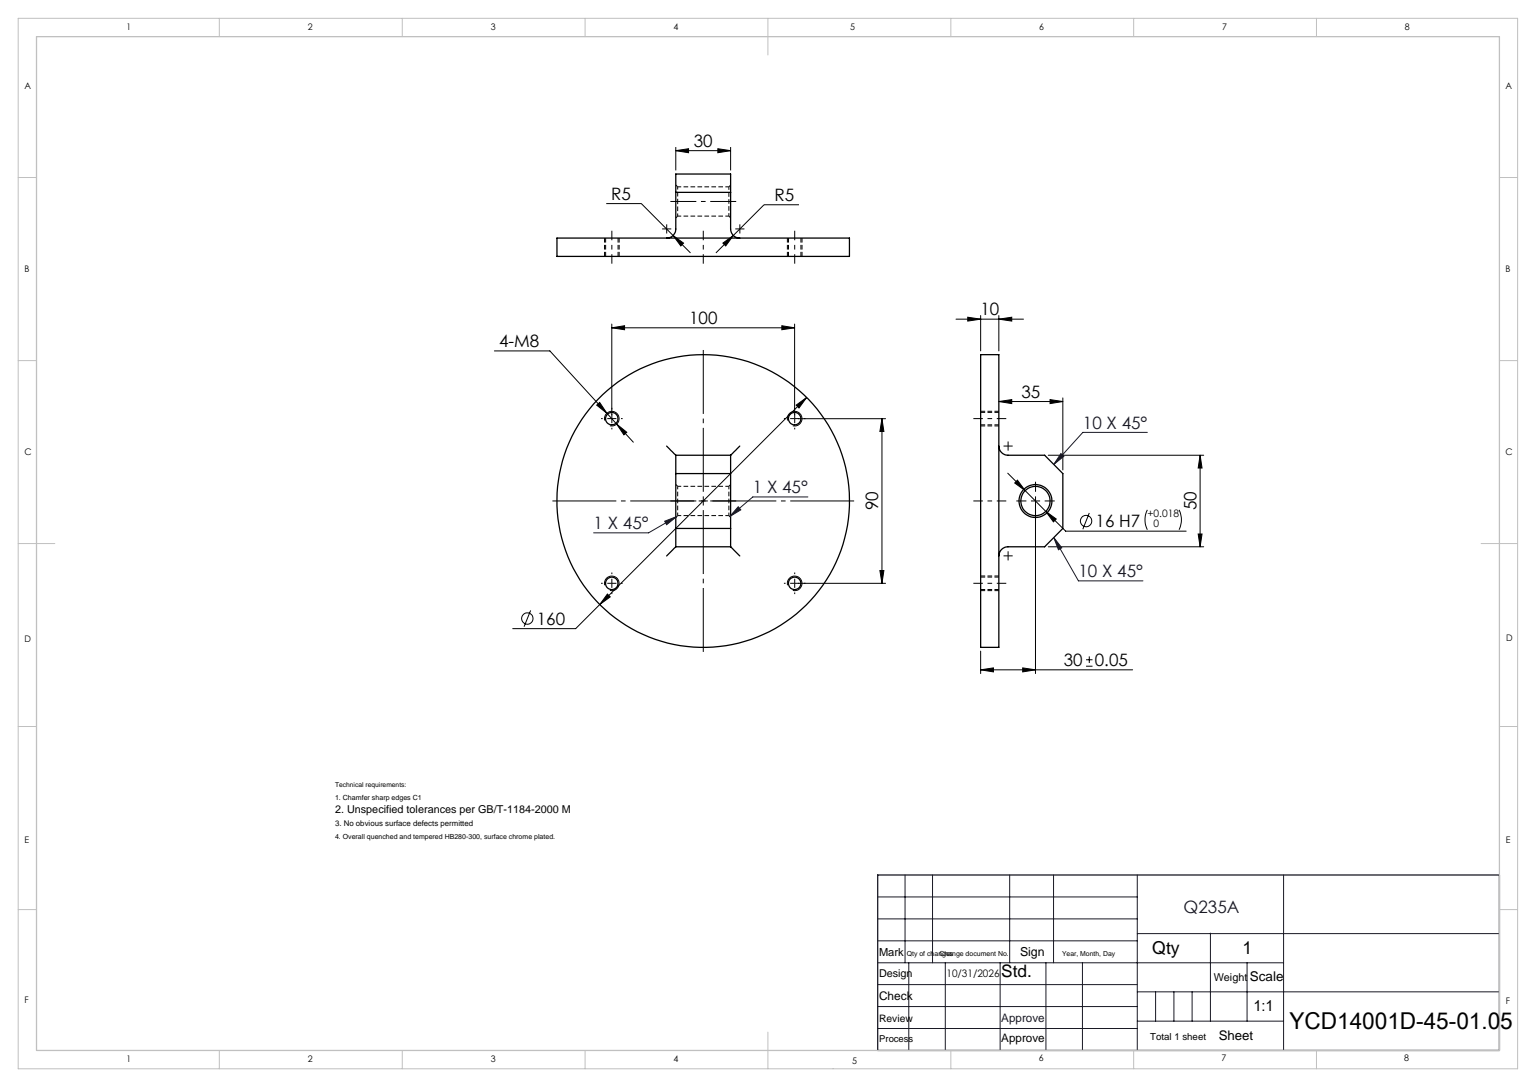
SolidWorks part; units mm, degrees
material "Q235A"
ref_plane "Front Plane" through (0, 0, 0) normal (0, 0, 1) x (1, 0, 0)
ref_plane "Top Plane" through (0, 0, 0) normal (0, 1, 0) x (1, 0, 0)
ref_plane "Right Plane" through (0, 0, 0) normal (1, 0, 0) x (0, 0, -1)
sketch "Sketch1" plane through (0, 0, 0) normal (0, 1, 0) x (1, 0, 0)
  circle A0 centre (0, 0) radius 80
  point P0 (0, 0)
  dimension "D1" = 160
extrude "Boss-Extrude1" add sketch "Sketch1" along normal mid plane 10
hole_wizard "M8 Tapped Hole1" positions "Sketch5" profile "Sketch4" tap size "M8" standard "Iso" end condition through all
sketch "Sketch5" plane through (0, -5, 0) normal (0, -1, 0) x (-1, 0, 0)
  line L0 (0, 0) -> (120.8477, 0) construction
  line L2 (0, 0) -> (0, -116.2317) construction
  point P0 (50, -45)
  point P13 (50, 45)
  point P14 (-50, 45)
  point P15 (-50, -45)
  dimension "D1" = 100
  dimension "D2" = 90
sketch "Sketch4" plane through (-50, -5, 45) normal (1, 0, 0) x (0, 0, -1)
  line L0 (0, 0) -> (0, 10)
  line L1 (0, 10) -> (3.4, 10)
  line L2 (3.4, 10) -> (3.4, 0)
  line L5 (3.4, 0) -> (0, 0)
  line L11 (0, -6.35) -> (0, 107.95) construction
  dimension "通孔螺纹孔钻头直径" = 6.8
  dimension "通孔螺纹孔钻头深度" = 10
cosmetic thread "Cosmetic Thread1" parameters "D1"=50, "D2"=8
cosmetic thread "Cosmetic Thread2" parameters "D1"=50, "D2"=8
cosmetic thread "Cosmetic Thread3" parameters "D1"=50, "D2"=8
cosmetic thread "Cosmetic Thread4" parameters "D1"=50, "D2"=8
sketch "Sketch6" plane through (0, 5, 0) normal (0, 1, 0) x (1, 0, 0)
  line L0 (-90, 57.5) -> (-90, 42.5) construction
  line L1 (-85.75, 57.5) -> (-85.75, 42.5)
  line L2 (-94.25, 57.5) -> (-94.25, 42.5)
  line L3 (90, 57.5) -> (90, 42.5) construction
  line L4 (94.25, 57.5) -> (94.25, 42.5)
  line L5 (85.75, 57.5) -> (85.75, 42.5)
  line L6 (0, 0) -> (135.0586, 0) construction
  line L7 (0, 0) -> (0, 102.7006) construction
  line L8 (90, -57.5) -> (90, -42.5) construction
  line L9 (94.25, -57.5) -> (94.25, -42.5)
  line L10 (85.75, -57.5) -> (85.75, -42.5)
  line L11 (-90, -57.5) -> (-90, -42.5) construction
  line L12 (-85.75, -57.5) -> (-85.75, -42.5)
  line L13 (-94.25, -57.5) -> (-94.25, -42.5)
  line L15 (10, 32.5) -> (-10, 32.5) construction
  arc A0 (-85.75, 57.5) -> (-94.25, 57.5) centre (-90, 57.5) ccw
  arc A1 (-94.25, 42.5) -> (-85.75, 42.5) centre (-90, 42.5) ccw
  arc A2 (94.25, 57.5) -> (85.75, 57.5) centre (90, 57.5) ccw
  arc A3 (85.75, 42.5) -> (94.25, 42.5) centre (90, 42.5) ccw
  arc A4 (94.25, -57.5) -> (85.75, -57.5) centre (90, -57.5) cw
  arc A5 (85.75, -42.5) -> (94.25, -42.5) centre (90, -42.5) cw
  arc A6 (-85.75, -57.5) -> (-94.25, -57.5) centre (-90, -57.5) cw
  arc A7 (-94.25, -42.5) -> (-85.75, -42.5) centre (-90, -42.5) cw
  point P2 (-90, 50)
  point P10 (90, 50)
  point P22 (90, -50)
  point P30 (-90, -50)
  dimension "D1" = 180
  dimension "D2" = 100
  dimension "D3" = 15
  dimension "D4" = 8.5
extrude "Cut-Extrude3" [suppressed] cut sketch "Sketch6" against normal blind 20
fillet "Fillet2" [suppressed] radius 10
sketch "Sketch7" plane through (0, -5, 0) normal (0, -1, 0) x (1, 0, 0)
  line L1 (-15, 25) -> (15, 25)
  line L2 (-15, 25) -> (-15, -25)
  line L3 (-15, -25) -> (15, -25)
  line L4 (15, 25) -> (15, -25)
  line L5 (-15, 25) -> (15, -25) construction
  line L6 (-15, -25) -> (15, 25) construction
  point P0 (0, 0)
  dimension "D1" = 30
  dimension "D2" = 50
extrude "Boss-Extrude2" add sketch "Sketch7" along normal blind 35
sketch "Sketch8" plane through (15, 0, 0) normal (1, 0, 0) x (0, 0, -1)
  circle A0 centre (0, -25) radius 8
  dimension "D1" = 16
  dimension "D2" = 25
extrude "Cut-Extrude4" cut sketch "Sketch8" against normal through all
chamfer "Chamfer1" distance 10 angle 45 2 edges at (0, -40, -25) (0, -40, 25)
fillet "Fillet3" radius 5 4 edges at (0, -5, -25) (15, -5, 0) (0, -5, 25) (-15, -5, 0)
chamfer "Chamfer2" distance 1 angle 45 2 edges at (-15, -25, -8) (15, -25, -8)
